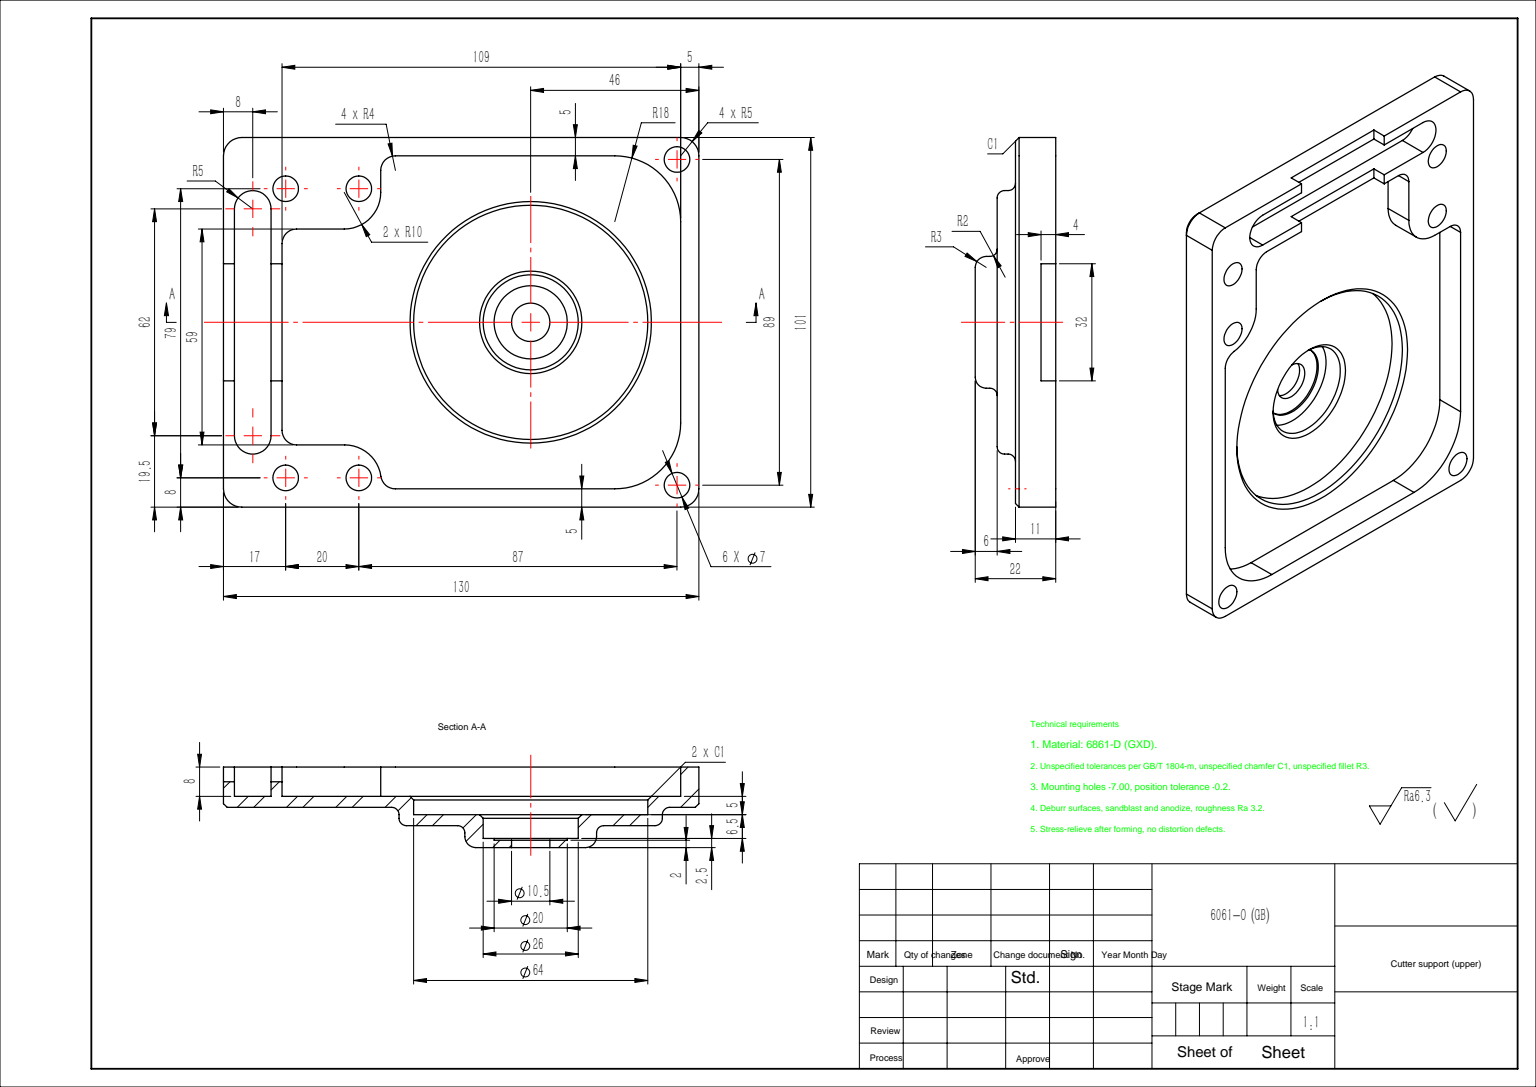
from build123d import *

# Parameters (mm, degrees)
SKETCH_1_W                = 101
SKETCH_1_H                = 130
EXTRUDE_1_DEPTH           = 11
CUT_EXTRUDE_1_DEPTH       = 8
CUT_EXTRUDE_2_DEPTH       = 8
CUT_EXTRUDE_3_REACH       = 1271.625
SKETCH_4_W                = 4
SKETCH_4_H                = 32
CUT_EXTRUDE_4_REACH       = 1273.161
SKETCH_5_W                = 4
SKETCH_5_H                = 32
SKETCH_6_R                = 36
EXTRUDE_2_DEPTH           = 5
SKETCH_7_R                = 18
EXTRUDE_3_DEPTH           = 6
SKETCH_8_R                = 32
CUT_EXTRUDE_5_DEPTH       = 5
SKETCH_9_R                = 13
CUT_EXTRUDE_6_DEPTH       = 6.5
SKETCH_10_R               = 10
CUT_EXTRUDE_7_DEPTH       = 0.5
SKETCH_11_R               = 5.25
CUT_EXTRUDE_8_DEPTH       = 97.916510461
HOLE_WIZARD_7_0_7_1_D     = 7
HOLE_WIZARD_7_0_7_1_DEPTH = 22
FILLET_1_R                = 5
CHAMFER_1_SIZE            = 1
FILLET_2_R                = 2
FILLET_3_R                = 3
FILLET_4_R                = 4
FILLET_5_R                = 10


with BuildPart() as part:
    # 草图1 → 凸台-拉伸1 (new body)
    with BuildSketch(Plane(origin=(1263, 0, 0), x_dir=(0, 0, -1), z_dir=(1, 0, 0))):
        with Locations((-11, -6.6)):
            Rectangle(SKETCH_1_W, SKETCH_1_H)
    extrude(amount=-EXTRUDE_1_DEPTH)

    # 草图2 → 切除-拉伸1 (cut)
    with BuildSketch(Plane(origin=(1263, 0, 0), x_dir=(0, 0, -1), z_dir=(1, 0, 0))):
        with BuildLine():
            Line((14.5, 42.4), (-44.5, 42.4))
            Line((-44.5, 42.4), (-44.5, 25.256406461))
            ThreePointArc((-44.5, 25.256406461), (-48.17544468, 17.510439768), (-56.5, 15.458447489))
            Line((-56.5, 15.458447489), (-56.5, -48.6))
            ThreePointArc((-56.5, -48.6), (-51.227922061, -61.327922061), (-38.5, -66.6))
            Line((-38.5, -66.6), (16.5, -66.6))
            ThreePointArc((16.5, -66.6), (29.227922061, -61.327922061), (34.5, -48.6))
            Line((34.5, -48.6), (34.5, 15.4))
            Line((34.5, 15.4), (14.5, 15.4))
            Line((14.5, 15.4), (14.5, 42.4))
        make_face()
    extrude(amount=-CUT_EXTRUDE_1_DEPTH, mode=Mode.SUBTRACT)

    # 草图3 → 切除-拉伸2 (cut)
    with BuildSketch(Plane(origin=(1263, 0, 0), x_dir=(0, 0, -1), z_dir=(1, 0, 0))):
        with BuildLine():
            Line((20, 55.4), (-42, 55.4))
            ThreePointArc((-42, 55.4), (-47, 50.4), (-42, 45.4))
            Line((-42, 45.4), (20, 45.4))
            ThreePointArc((20, 45.4), (25, 50.4), (20, 55.4))
        make_face()
    extrude(amount=-CUT_EXTRUDE_2_DEPTH, mode=Mode.SUBTRACT)

    # 草图4 → 切除-拉伸3 (cut, up to next)
    with BuildSketch(Plane.XZ.offset(-42.4), mode=Mode.PRIVATE) as cut_extrude_3_sk1:
        with Locations((1261, 11)):
            Rectangle(SKETCH_4_W, SKETCH_4_H)
    cut_extrude_3_tool1 = extrude(cut_extrude_3_sk1.sketch, amount=-CUT_EXTRUDE_3_REACH, mode=Mode.PRIVATE) & part.part
    add(cut_extrude_3_tool1.solids().sort_by_distance((1261, 42.4, 11))[0], mode=Mode.SUBTRACT)

    # 草图5 → 切除-拉伸4 (cut, up to next)
    with BuildSketch(Plane(origin=(0, 58.4, 0), x_dir=(-1, 0, 0), z_dir=(0, 1, 0)), mode=Mode.PRIVATE) as cut_extrude_4_sk1:
        with Locations((-1261, 11)):
            Rectangle(SKETCH_5_W, SKETCH_5_H)
    cut_extrude_4_tool1 = extrude(cut_extrude_4_sk1.sketch, amount=-CUT_EXTRUDE_4_REACH, mode=Mode.PRIVATE) & part.part
    add(cut_extrude_4_tool1.solids().sort_by_distance((1261, 58.4, 11))[0], mode=Mode.SUBTRACT)

    # 草图6 → 凸台-拉伸2 (add)
    with BuildSketch(Plane.ZY.offset(-1252)):
        with Locations((11, -25.6)):
            Circle(SKETCH_6_R)
    extrude(amount=EXTRUDE_2_DEPTH)

    # 草图7 → 凸台-拉伸3 (add)
    with BuildSketch(Plane.ZY.offset(-1247)):
        with Locations((11, -25.6)):
            Circle(SKETCH_7_R)
    extrude(amount=EXTRUDE_3_DEPTH)

    # 草图8 → 切除-拉伸5 (cut)
    with BuildSketch(Plane(origin=(1255, 0, 0), x_dir=(0, 0, -1), z_dir=(1, 0, 0))):
        with Locations(Location((-11, -25.6, 0), (0, 0, 180))):
            Circle(SKETCH_8_R)
    extrude(amount=-CUT_EXTRUDE_5_DEPTH, mode=Mode.SUBTRACT)

    # 草图9 → 切除-拉伸6 (cut)
    with BuildSketch(Plane(origin=(1250, 0, 0), x_dir=(0, 0, -1), z_dir=(1, 0, 0))):
        with Locations(Location((-11, -25.6, 0), (0, 0, 180))):
            Circle(SKETCH_9_R)
    extrude(amount=-CUT_EXTRUDE_6_DEPTH, mode=Mode.SUBTRACT)

    # 草图10 → 切除-拉伸7 (cut)
    with BuildSketch(Plane(origin=(1243.5, 0, 0), x_dir=(0, 0, -1), z_dir=(1, 0, 0))):
        with Locations(Location((-11, -25.6, 0), (0, 0, 180))):
            Circle(SKETCH_10_R)
    extrude(amount=-CUT_EXTRUDE_7_DEPTH, mode=Mode.SUBTRACT)

    # 草图11 → 切除-拉伸8 (cut, through all)
    with BuildSketch(Plane.ZY.offset(-1241)):
        with Locations((11, -25.6)):
            Circle(SKETCH_11_R)
    extrude(amount=-CUT_EXTRUDE_8_DEPTH, mode=Mode.SUBTRACT)

    # Ø7.0 (7) 直径孔1
    with Locations(Plane(origin=(1263, 0, 0), x_dir=(0, 0, -1), z_dir=(1, 0, 0))):
        with Locations((-55.5, -65.6), (33.5, -65.6), (25.5, 21.4), (25.5, 41.4), (-53.5, 41.4), (-53.5, 21.4)):
            Hole(HOLE_WIZARD_7_0_7_1_D / 2, depth=HOLE_WIZARD_7_0_7_1_DEPTH)

    # 圆角1
    fillet_1_edges = [part.edges().sort_by_distance(p)[0] for p in [
        (1257.5, -71.6, -39.5),
        (1257.5, -71.6, 61.5),
        (1257.5, 58.4, 61.5),
        (1257.5, 58.4, -39.5),
    ]]
    fillet(fillet_1_edges, radius=FILLET_1_R)

    # 倒角1
    chamfer_1_edges = [part.edges().sort_by_distance(p)[0] for p in [
        (1252, 58.4, 11),
        (1252, -6.6, 61.5),
        (1252, -6.6, -39.5),
        (1252, -71.6, 11),
        (1252, -70.135533906, 60.035533906),
        (1252, -70.135533906, -38.035533906),
        (1252, 56.935533906, -38.035533906),
        (1252, 56.935533906, 60.035533906),
        (1255, -25.6, -21),
        (1250, -25.6, -2),
    ]]
    chamfer(chamfer_1_edges, length=CHAMFER_1_SIZE)

    # 圆角2
    fillet_2_edges = [part.edges().sort_by_distance(p)[0] for p in [
        (1252, -25.6, -25),
        (1247, -25.6, -25),
        (1247, -25.6, -7),
    ]]
    fillet(fillet_2_edges, radius=FILLET_2_R)

    # 圆角3
    fillet_3_edges = [part.edges().sort_by_distance(p)[0] for p in [
        (1241, -25.6, -7),
    ]]
    fillet(fillet_3_edges, radius=FILLET_3_R)

    # 圆角4
    fillet_4_edges = [part.edges().sort_by_distance(p)[0] for p in [
        (1259, 42.4, -14.5),
        (1259, 15.4, -34.5),
        (1259, 15.458447489, 56.5),
        (1259, 42.4, 44.5),
    ]]
    fillet(fillet_4_edges, radius=FILLET_4_R)

    # 圆角5
    fillet_5_edges = [part.edges().sort_by_distance(p)[0] for p in [
        (1259, 15.4, -14.5),
    ]]
    fillet(fillet_5_edges, radius=FILLET_5_R)


solid = part.part
